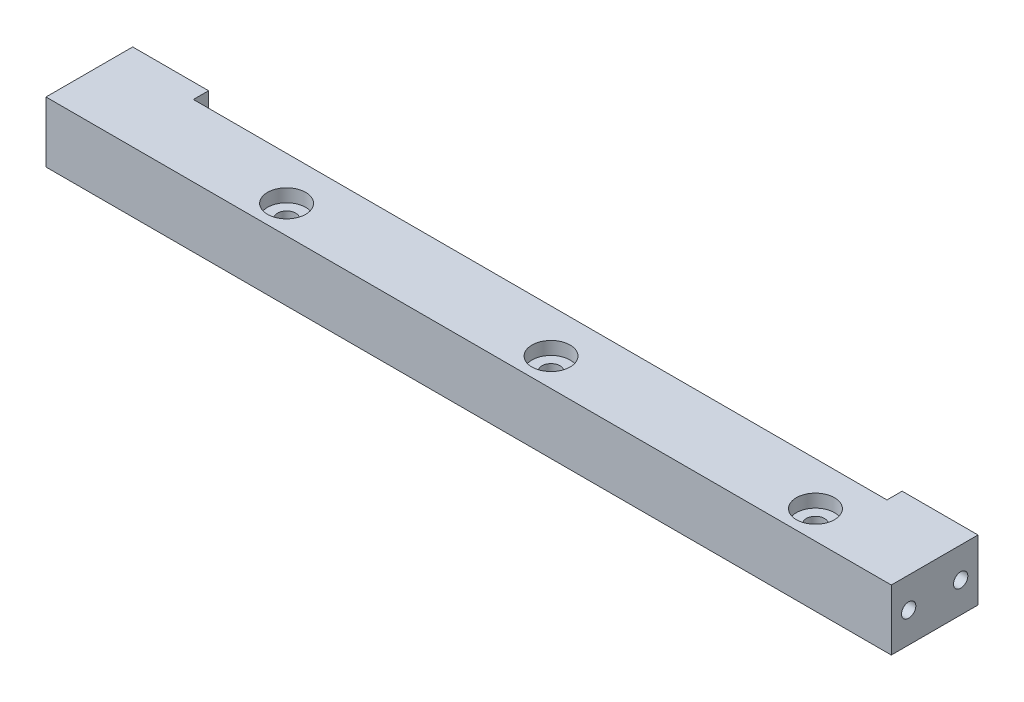
from build123d import *

# Parameters (mm, degrees)
SKETCH1_W             = 195
SKETCH1_H             = 14
EXTRUDE_THIN1_DEPTH   = 10
M4_TAPPED_HOLE1_D     = 3.3
M4_TAPPED_HOLE1_DEPTH = 10.1
M4_TAPPED_HOLE1_TIP   = 0.991420021
M4_TAPPED_HOLE2_D     = 3.3
M4_TAPPED_HOLE2_DEPTH = 10.1
M4_TAPPED_HOLE2_TIP   = 0.991420021
M5_TAPPED_HOLE1_D     = 4.2
SKETCH9_R             = 4.4
CUT_EXTRUDE1_DEPTH    = 3
SKETCH10_W            = 160
SKETCH10_H            = 3.5
CUT_EXTRUDE2_DEPTH    = 196.757503049


with BuildPart() as part:
    # Sketch1 → Extrude-Thin1 (new, symmetric)
    with BuildSketch(Plane.XY):
        with Locations((-97.5, 7)):
            Rectangle(SKETCH1_W, SKETCH1_H)
    extrude(amount=EXTRUDE_THIN1_DEPTH, both=True)

    # M4 Tapped Hole1
    with Locations(Plane.ZY.offset(195)):
        with Locations((-6, 7), (6, 7)):
            Hole(M4_TAPPED_HOLE1_D / 2, depth=M4_TAPPED_HOLE1_DEPTH)
            with Locations((0, 0, -(M4_TAPPED_HOLE1_DEPTH + M4_TAPPED_HOLE1_TIP / 2))):  # 118° drill point
                Cone(0, M4_TAPPED_HOLE1_D / 2, M4_TAPPED_HOLE1_TIP, mode=Mode.SUBTRACT)

    # M4 Tapped Hole2
    with Locations(Plane(origin=(0, 0, 0), x_dir=(0, 0, -1), z_dir=(1, 0, 0))):
        with Locations((-6, 7), (6, 7)):
            Hole(M4_TAPPED_HOLE2_D / 2, depth=M4_TAPPED_HOLE2_DEPTH)
            with Locations((0, 0, -(M4_TAPPED_HOLE2_DEPTH + M4_TAPPED_HOLE2_TIP / 2))):  # 118° drill point
                Cone(0, M4_TAPPED_HOLE2_D / 2, M4_TAPPED_HOLE2_TIP, mode=Mode.SUBTRACT)

    # M5 Tapped Hole1 (through all)
    with Locations(Plane(origin=(0, 14, 0), x_dir=(1, 0, 0), z_dir=(0, 1, 0))):
        with Locations((-146, -3.5), (-85, -3.5), (-24, -3.5)):
            Hole(M5_TAPPED_HOLE1_D / 2)

    # Sketch9 → Cut-Extrude1 (cut)
    with BuildSketch(Plane(origin=(0, 14, 0), x_dir=(1, 0, 0), z_dir=(0, 1, 0))):
        with Locations(Location((-146, -3.5, 0), (0, 0, 180))):
            Circle(SKETCH9_R)
        with Locations(Location((-85, -3.5, 0), (0, 0, 180))):
            Circle(SKETCH9_R)
        with Locations(Location((-24, -3.5, 0), (0, 0, 180))):
            Circle(SKETCH9_R)
    extrude(amount=-CUT_EXTRUDE1_DEPTH, mode=Mode.SUBTRACT)

    # Sketch10 → Cut-Extrude2 (cut, through all)
    with BuildSketch(Plane(origin=(0, 14, 0), x_dir=(1, 0, 0), z_dir=(0, 1, 0))):
        with Locations((-97.5, 8.25)):
            Rectangle(SKETCH10_W, SKETCH10_H)
    extrude(amount=-CUT_EXTRUDE2_DEPTH, mode=Mode.SUBTRACT)


solid = part.part
